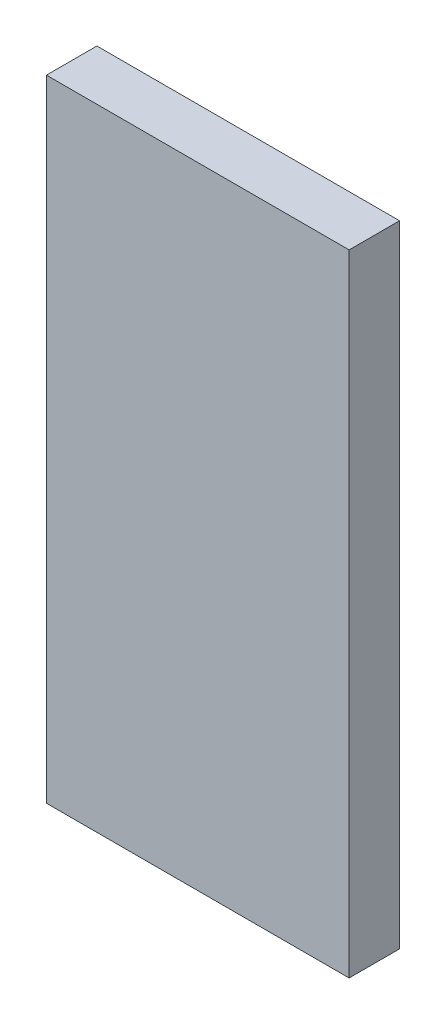
SolidWorks part; units mm, degrees
material "普通碳钢"
ref_plane "Front Plane" through (0, 0, 0) normal (0, 0, 1) x (1, 0, 0)
ref_plane "Top Plane" through (0, 0, 0) normal (0, 1, 0) x (1, 0, 0)
ref_plane "Right Plane" through (0, 0, 0) normal (1, 0, 0) x (0, 0, -1)
sketch "Sketch1" plane through (0, 0, 0) normal (0, 0, 1) x (1, 0, 0)
  line L2 (48, 100) -> (-48, 100)
  line L3 (-48, 100) -> (-48, -100)
  line L4 (-48, -100) -> (48, -100)
  line L5 (48, -100) -> (48, 100)
  dimension "D1" = 200
  dimension "D2" = 96
extrude "Extrude1" add sketch "Sketch1" along normal mid plane 16
ref_plane "Plane1" through (36, 0, 0) normal (1, 0, 0) x (0, 0, -1)
ref_plane "Plane2" through (-36, 0, 0) normal (-1, 0, 0) x (0, 0, 1)
